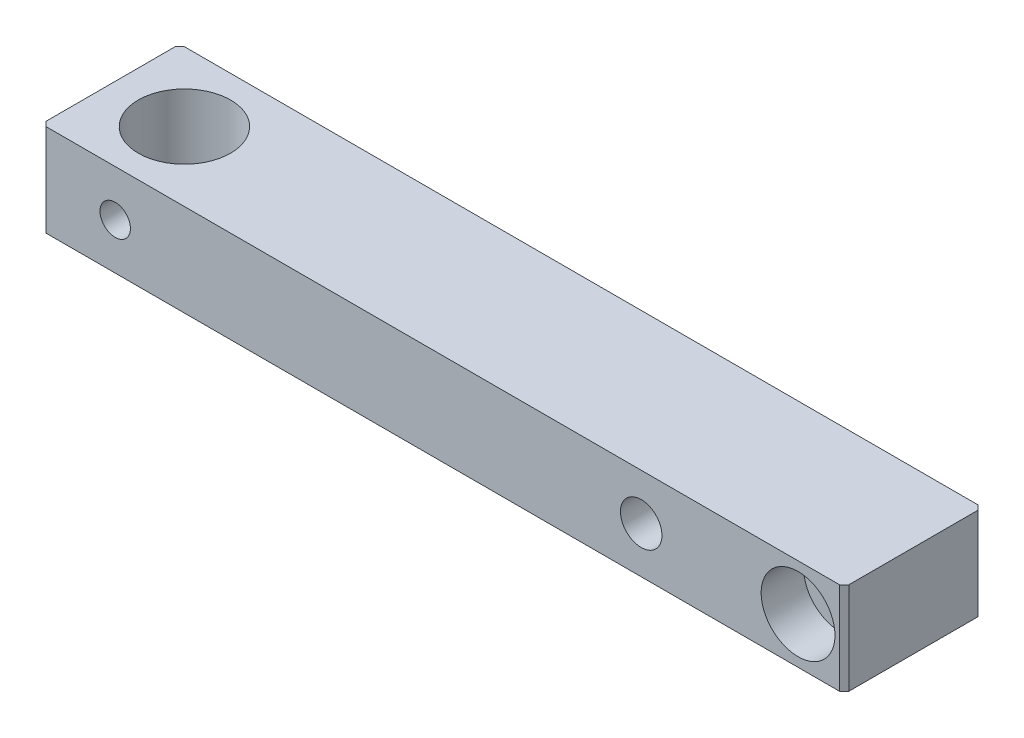
from build123d import *

# Parameters (mm, degrees)
SKETCH1_W                                            = 87
SKETCH1_H                                            = 15
BOSS_EXTRUDE1_DEPTH                                  = 10
SKETCH2_R                                            = 5
CUT_EXTRUDE1_DEPTH                                   = 46.260357931
F_4_5_4_5_DIAMETER_HOLE2_D                           = 4.5
CBORE_FOR_M4_SLOTTED_CHEESE_HEAD_SCREWS2_D           = 4.5
CBORE_FOR_M4_SLOTTED_CHEESE_HEAD_SCREWS2_CBORE_D     = 8
CBORE_FOR_M4_SLOTTED_CHEESE_HEAD_SCREWS2_CBORE_DEPTH = 4.6
CHAMFER1_SIZE                                        = 0.5
M4_TAPPED_HOLE2_D                                    = 3.3
M4_TAPPED_HOLE2_DEPTH                                = 8
M4_TAPPED_HOLE2_TIP                                  = 0.991420021


with BuildPart() as part:
    # Sketch1 → Boss-Extrude1 (new body)
    with BuildSketch(Plane(origin=(0, 0, 0), x_dir=(1, 0, 0), z_dir=(0, 1, 0))):
        Rectangle(SKETCH1_W, SKETCH1_H)
    extrude(amount=BOSS_EXTRUDE1_DEPTH)

    # Sketch2 → Cut-Extrude1 (cut, through all)
    with BuildSketch(Plane(origin=(0, 10, 0), x_dir=(1, 0, 0), z_dir=(0, 1, 0))):
        with Locations(Location((-35.5, 0, 0), (0, 0, 270))):
            Circle(SKETCH2_R)
    extrude(amount=-CUT_EXTRUDE1_DEPTH, mode=Mode.SUBTRACT)

    # Ø4.5 (4.5) Diameter Hole2 (through all)
    with Locations(Plane(origin=(0, 0, -7.5), x_dir=(-1, 0, 0), z_dir=(0, 0, -1))):
        with Locations((-21.5, 5)):
            Hole(F_4_5_4_5_DIAMETER_HOLE2_D / 2)

    # CBORE for M4 Slotted cheese head screws2 (through all)
    with Locations(Plane.XY.offset(7.5)):
        with Locations((38.5, 5)):
            CounterBoreHole(CBORE_FOR_M4_SLOTTED_CHEESE_HEAD_SCREWS2_D / 2, CBORE_FOR_M4_SLOTTED_CHEESE_HEAD_SCREWS2_CBORE_D / 2, CBORE_FOR_M4_SLOTTED_CHEESE_HEAD_SCREWS2_CBORE_DEPTH)

    # Chamfer1
    chamfer1_edges = [part.edges().sort_by_distance(p)[0] for p in [
        (-43.5, 5, -7.5),
        (43.5, 5, -7.5),
        (43.5, 5, 7.5),
        (-43.5, 5, 7.5),
    ]]
    chamfer(chamfer1_edges, length=CHAMFER1_SIZE)

    # M4 Tapped Hole2
    with Locations(Plane.XY.offset(7.5)):
        with Locations((-35.5, 5)):
            Hole(M4_TAPPED_HOLE2_D / 2, depth=M4_TAPPED_HOLE2_DEPTH)
            with Locations((0, 0, -(M4_TAPPED_HOLE2_DEPTH + M4_TAPPED_HOLE2_TIP / 2))):  # 118° drill point
                Cone(0, M4_TAPPED_HOLE2_D / 2, M4_TAPPED_HOLE2_TIP, mode=Mode.SUBTRACT)


solid = part.part
